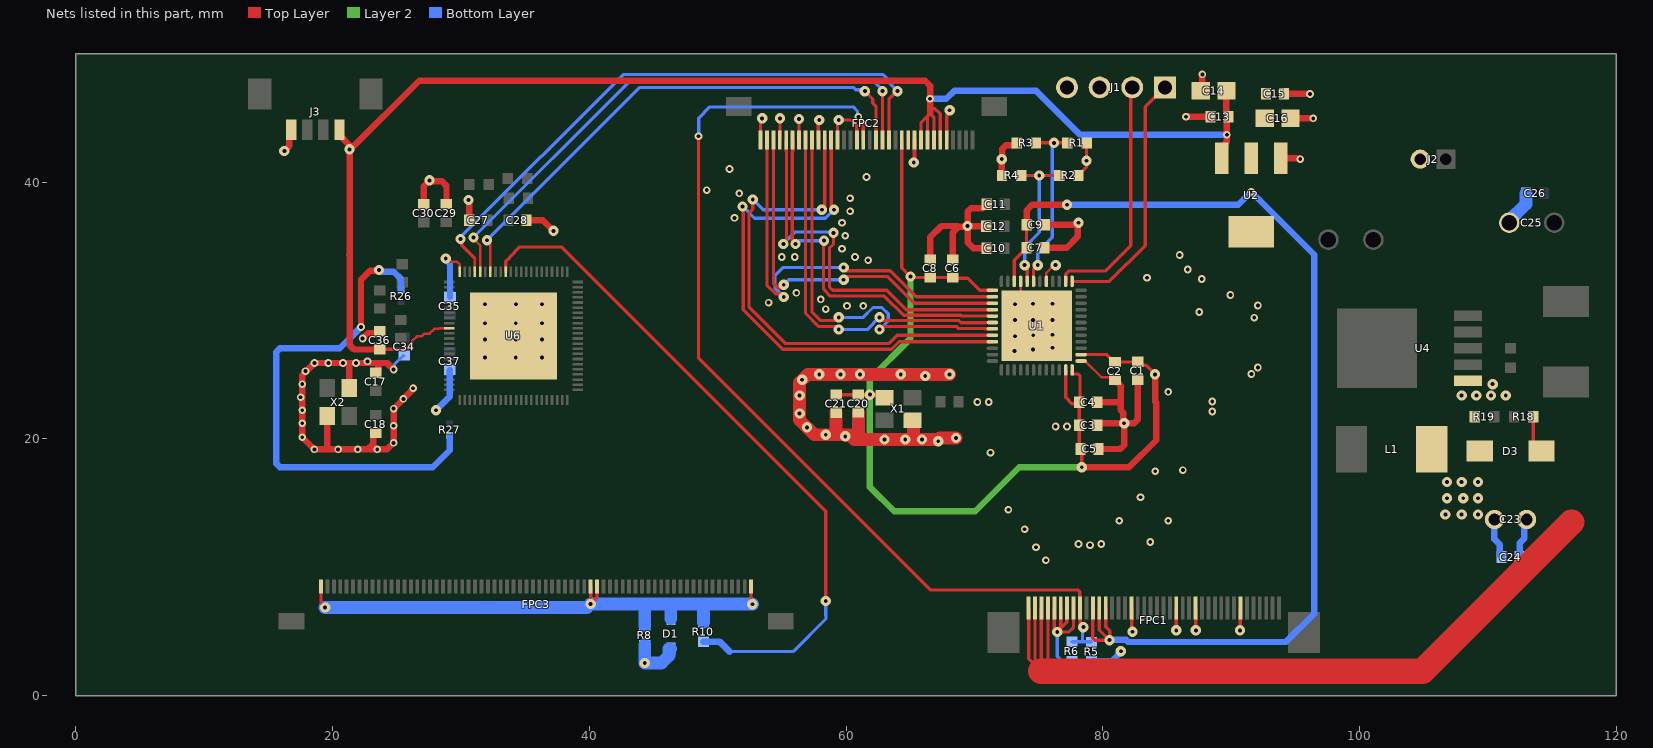
[diagram p0: the nets of this part, all layers, seen from the top]
# Altium PCB MISC71201-3.PcbDoc (part 2 of 3)
Units mm, origin at the board's own origin, x right, y up, seen from the top; angles counter-clockwise.
Board outline 120 x 50 mm, 4 copper layers (Top Layer, Layer 1, Layer 2, Bottom Layer), stack 0.603 mm thick; 69 components, 139 nets, 430 pads, 271 vias.

## Part data (continued)
C23: "Capacitance:220uF;Tolerance:±20%;Rated voltage:25V;Ripple current:510mA@100kHz;Equivalent series resistance (ESR):130mΩ@100kHz;", Equivalent Series Resistance(ESR)=130mΩ@100kHz, JLCPCB Part Class="Extended Part", LCSC Part Name="220uF ±20% 25V", Manufacturer=JIERR(捷而瑞), ManufacturerPart=ERG25V220M6X11, Operating Temperature=-40℃~+105℃, Ripple Current=510mA@100kHz, Tolerance=±20%, Voltage Rating=25V
C27: library part C0402_1u_6.3V_X5R, "SMD capacitor", PartNumber=00226021661, Value1=0.1uF/6.3V, Value2=X5R
C28 C34 C35 C36 C37: library part C0402_2.2u_6.3V_X5R, "SMD capacitor", PartNumber=002260222561, Value1=1uF/6.3V, Value2=X5R
C29 C30: library part C0603_1u_50V_X7R, "SMD capacitor", PartNumber=002260310544, Value1=4.7uF/50V, Value2=X7R
C31 C32 C33: library part C0603_1u_50V_X7R, "SMD capacitor", PartNumber=002260310544, Value1=1uF/50V, Value2=X7R
D1: library part pdyl240b_c5187140, "Reverse standoff voltage (Vrwm):24V;Clamping voltage:60V;Peak pulse power (Ppp):350W@8/20us;Breakdown voltage (VBR):26.7V;", Clamping Voltage=60V, JLCPCB Part Class="Extended Part", Junction Capacitance=1pF, LCSC Part Name="ESD 24V截止", Manufacturer=Leiditech(雷卯电子), ManufacturerPart=PDYL240B, Peak Pulse Power Dissipation (Ppp)=350W@8/20us, Reverse Leakage Current (Ir)=1uA, Reverse Stand-Off Voltage (Vrwm)=24V, Voltage - Breakdown=26.7V
D3: library part ss34_c7420365, "Diode configuration:Single;Forward voltage (Vf):550mV@3A;DC reverse voltage (Vr):40V;Rectified current:3A;", Current - Rectified=3A, JLCPCB Part Class="Extended Part", LCSC Part Name="电压:40V 电流:3A", Manufacturer=R+O(宏嘉诚), ManufacturerPart=SS34, Reverse Leakage Current (Ir)=200uA@40V, Voltage - DC Reverse(Vr)=40V, Voltage - Forward(Vf@If)=550mV@3A
FPC1: "Locking:Slide;Contact type:Bottom;Contacts:40P;Pitch:0.5mm;Mounting:Horizontal SMT;Operating temperature:-25℃~+85℃;", JLCPCB Part Class="Extended Part", LCSC Part Name="间距:0.5mm 40P 抽屉式 下接", Manufacturer=BXCONN(宝讯), ManufacturerPart=FC-05D40P11H20, Operating Temperature=-25℃~+85℃, Rated Voltage (Max)=50V
FPC2: "Locking:Flip;Contact type:Bottom;Contacts:34P;Pitch:0.5mm;Mounting:Horizontal SMT;Operating temperature:-40℃~+85℃;", Current Rating (Max)=500mA, JLCPCB Part Class="Extended Part", LCSC Part Name="FPC 翻盖式 下接 P数:34P 间距:0.5mm", Manufacturer=BXCONN(宝讯), ManufacturerPart=FC-05A34P011H20, Operating Temperature=-40℃~+85℃, Rated Voltage (Max)=50V
FPC3: "Locking:Flip;Contact type:Bottom;Contacts:68P;Pitch:0.5mm;Mounting:Horizontal SMT;Operating temperature:-25℃~+85℃;", Current Rating (Max)=500mA, JLCPCB Part Class="Extended Part", LCSC Part Name="翻盖式 下接 P数:68P 间距:0.5mm", Manufacturer=JS(钜硕电子), ManufacturerPart=AFC18-S68FIA-00, Operating Temperature=-25℃~+85℃, Rated Voltage (Max)=50V
J1: "Pin structure:1x4P;Pitch:2.54mm;Row pitch:-;Round/square pin:Square;Mounting:THT;Rows:Single;Total pins:4P;Rated current:3A;Rated voltage:1kV;Mating pin length:6mm;Insulator height:2.5mm;Tail length:3mm;Contact material:Brass;Contact plating:Gold;Operating temperature:-40℃~+105℃;Color:Black;", Color=黑色, Current Rating=3A, JLCPCB Part Class="Extended Part", LCSC Part Name="1x4P 间距:2.54mm 方针 直插", Manufacturer=hanxia(韩下), ManufacturerPart="HX PZ2.54-1x4P ZZ", Operating Temperature=-40℃~+105℃, Voltage Rating (Max)=1kV
J2: "Pin structure:1x2P;Pitch:2mm;Mounting:Right-angle THT;Series:PA;Total pins:2P;Rows:1;Pins per row:2;Row pitch:-;Rated current:3A;Contact material:Copper alloy;Contact plating:Tin;Operating temperature:-25℃~+85℃;", Color=白色, Current Rating=3A, Flame Retardant Rating=UL94V-0, JLCPCB Part Class="Extended Part", LCSC Part Name="1x2P 间距:2mm 弯插 系列:PA", Manufacturer=JST, ManufacturerPart=S02B-PASK-2(LF)(SN), Operating Temperature=-25℃~+85℃, Voltage Rating=250V
J3: "Pin structure:1x4P;Pitch:1.25mm;Mounting:Horizontal SMT;Series:PicoBlade(MX 1.25);Total pins:4P;Rows:1;Pins per row:4;Rated current:1A;Contact material:Brass;Contact plating:Tin;Operating temperature:-25℃~+85℃;", Current Rating=1A, JLCPCB Part Class="Extended Part", LCSC Part Name="1x4P 间距:1.25mm 卧贴 系列:PicoBlade(MX 1.25)", Manufacturer=LXWCONN(连兴旺电子), ManufacturerPart=MX1.25mm-4P-WT, Operating Temperature=-25℃~+85℃, Voltage Rating=125V
L1 L2: "SMD, 7x6.6x2.8mm   alloy inductor, molded inductor, high current", JLCPCB Part Class="Extended Part", LCSC Part Name="15uH ±20%", Manufacturer=cjiang(长江微电), ManufacturerPart=FXL0630-150-M
R1 R2 R3 R4 R5 R6 R7: library part Resistor
R8 R10: library part Res2, POWER=0.1W, Tolerance=1%
R9 R25: library part Res2, "SMD resistor"
R18: "Resistor type:Thin film;Resistance:86.6kΩ;Tolerance:±0.1%;Power:100mW;Temp. coefficient:±25ppm/℃;", JLCPCB Part Class="Extended Part", LCSC Part Name="薄膜电阻 86.6kΩ ±0.1% 100mW", Manufacturer=YAGEO(国巨), ManufacturerPart=RT0603BRD0786K6L, Operating Temperature Range=-55℃~+155℃, Power(Watts)=100mW, Temperature Coefficient=±25ppm/℃, Tolerance=±0.1%
R19 R20: "Resistor type:Thin film;Resistance:10kΩ;Tolerance:±0.1%;Power:100mW;Operating voltage:75V;Temp. coefficient:±25ppm/℃;", JLCPCB Part Class="Extended Part", LCSC Part Name="薄膜电阻 10kΩ ±0.1% 100mW", Manufacturer=YAGEO(国巨), ManufacturerPart=RT0603BRD0710KL, Operating Temperature=-55℃~+155℃, Power(Watts)=100mW, Temperature Coefficient=±25ppm/℃, Tolerance=±0.1%, Voltage-Supply(Max)=75V
R26 R27: library part R0402_0R_+-5%_Dup2, "SMD resistor", PartNumber=00105020003, Value1=0R, Value2=∮5%
U1: library part stm32f411ceu6, "CPU core:ARM Cortex-M4;CPU max frequency:100MHz;CPU bits:32 Bit;", JLCPCB Part Class="Extended Part", LCSC Part Name="带DSP和FPU的高性能基本型系列ARM Cortex-M4 MCU，具有512 KB Flash、100 MHz CPU和ART加速器", Manufacturer=ST(意法半导体), ManufacturerPart=STM32F411CEU6, Operating Temperature=-40℃~+85℃, Voltage - Supply=1.7V~3.6V
U2: "Output polarity:Positive;Operating voltage:12V;Output voltage:3.3V;Output current:1A;PSRR:60dB@(120Hz);Output type:Fixed;", JLCPCB Part Class="Extended Part", LCSC Part Name="3.3V 1A 12V", Manufacturer=BL(上海贝岭), ManufacturerPart=BL1117-33CX, Operating Temperature=-20℃~+125℃@(Tj), Output Current=1A, Output Voltage=3.3V, Power Supply Rejection Ratio (PSRR)=60dB@(120Hz), standby current=2mA, Voltage - Supply=12V, Voltage Dropout=1.5V@(1A)
U4: "Function:Buck-boost;Operating voltage:3.6V~32V;Output voltage:-;Output current:3A;Output type:Adjustable;", Frequency - Switching=320kHz~480kHz, JLCPCB Part Class="Extended Part", LCSC Part Name="升降压型 3A 3.6V~32V", Manufacturer=XLSEMI(芯龙), ManufacturerPart=XL6008E1, Operating Temperature=-40℃~+125℃@(TJ), Output Current=3A, Output Voltage=-, Quiescent Current=2.5mA, Voltage - Supply=3.6V~32V
U6: library part ILI2511/QFN-88/10X10_0.4_0.9, "ILITEK IC", Part Name=005122ILI2511
X1: "Frequency:26MHz;Frequency tolerance (room temp.):±10ppm;Output:CMOS;Operating voltage:1.8V~3.3V;Frequency stability:±20ppm;", Frequency Stability=±20ppm, JLCPCB Part Class="Extended Part", LCSC Part Name="YSO110TR 26MHZ 1.8V-3.3V ±10PPM -40~85℃（±20PPM) CMOS", Manufacturer=YXC(扬兴晶振), ManufacturerPart=OT322526MJBA4SL, Normal temperature Frequency Tolerance=±10ppm, Operating Temperature=-40℃~+85℃, Voltage - Supply=1.8V~3.3V
X2: "Crystal type:SMD crystal;Frequency:12MHz;Frequency tolerance (room temp.):±10ppm;Load capacitance:20pF;Frequency stability:±20ppm;", Equivalent Series Resistance(ESR)=80Ω, Frequency Stability=±20ppm, JLCPCB Part Class="Basic Part", LCSC Part Name="YSX321SL 12MHZ 4P 3225 20PF ±10PPM -40~85℃ (±20PPM)", Load Capacitance=20pF, Manufacturer=YXC(扬兴晶振), ManufacturerPart=X322512MSB4SI, Normal temperature Frequency Tolerance=±10ppm, Operating Temperature=-40℃~+85℃

## Via types
v1: diameter 0.8, hole 0.3, Top Layer to Bottom Layer, 182 vias
v2: diameter 0.6, hole 0.3, Top Layer to Bottom Layer, 89 vias

## Nets (pads, with @x,y where several pads share a name; then routed paths per layer and width w, separated by ;. In a path a pad name is that pad's centre, name@x,y a point inside that pad or via, vN(x,y) a via of type N, cw(c..) or ccw(c..) an arc to the next point about the centre after c; other vN are vias at no path point)
"1.8V for TFT": C1.2 C2.2 C3.2 C4.2 C5.1 C6.2 C8.2 C20.2 C21.2 FPC2.23 U1.13 U1.35 U1.36 U1.38 X1.4 | length 87.9
  Top Layer w0.254: C21.2@59.224,23.426 60.955,23.426 C20.2@60.97,23.442 v1(61.86,23.442) 62.75,23.442 X1.4@62.984,23.208 ; FPC2.23@64.345,43.277 64.345,33.318 v1(65.024,32.639) 65.09,32.573 C8.2@66.548,32.573 C6.2@68.326,32.573 68.387,32.512 69.469,32.512 70.419,31.562 U1.13@71.407,31.562 ; U1.35@77.107,25.362 77.107,23.223 77.597,22.733 78.051,22.733 C4.2@78.168,22.85 ; U1.36@77.608,25.362 77.608,25.059 77.62,25.047 78.077,25.047 78.232,24.892 78.232,22.914 C4.2@78.168,22.85 ; U1.38@78.306,26.561 80.321,26.561 80.9,25.982 C2.2@80.95,25.982 82.713,25.982 C1.2@82.728,25.997 83.001,25.724 83.369,25.724 v1(84.074,25.019) ; v1(78.359,17.78) 78.359,19.121 C5.1@78.273,19.207 78.174,19.307 C3.2@78.174,21.052 78.168,21.057 78.168,22.733 C4.2@78.168,22.85
  Top Layer w0.5: v1(78.359,17.78) 82.042,17.78 84.157,19.895 84.157,22.813 84.074,22.896 v1(84.074,25.019)
  Layer 2 w0.5: v1(65.024,32.639) 65.024,27.813 61.86,24.649 v1(61.86,23.442) 61.86,16.245 63.754,14.351 70.055,14.351 73.484,17.78 v1(78.359,17.78)
"3.3V for Touch&TFT": FPC2.25 J1.3 R1.1 R2.1 R5.1 R26.1 R27.1 | length 47
  Top Layer w0.254: R2.1@78.105,40.513 78.105,40.542 78.74,41.177 v1(78.74,41.656) R1.1@78.74,43.053
  Top Layer w0.3: v1(65.278,41.529) 65.345,41.596 FPC2.25@65.345,43.277
  Top Layer w0.5: v2(22.225,28.702) 22.225,32.385 22.93,33.09 23.565,33.09 v1(23.622,33.147)
  Bottom Layer w0.5: v2(22.225,28.702) 20.574,27.051 15.914,27.051 15.621,26.758 15.621,18.073 15.914,17.78 27.813,17.78 29.134,19.101 R27.1@29.134,20.262 ; v1(23.622,33.147) 23.749,33.02 24.765,33.02 25.342,32.443 R26.1@25.342,31.554 ; R5.1@79.121,2.667 80.772,2.667 80.772,2.739 81.407,3.374 v1(81.407,3.455)
"5V for BL": C13.1 C14.2 C36.2 FPC2.26 FPC2.27 FPC2.28 FPC2.29 J3.1 U2.3 U6.10 | length 115.3
  Top Layer w0.2: 25.84,27.14 26.209,27.509 26.209,27.602 26.59,27.983 26.948,27.983 27.159,28.194 27.572,28.194 27.943,28.565 28.342,28.565 28.392,28.615 U6.10@29.101,28.615
  Top Layer w0.254: C36.2@23.675,26.977 25.677,26.977 25.84,27.14 ; FPC2.26@65.845,43.277 65.845,44.636 66.345,45.136 ; FPC2.27@66.345,43.277 66.345,45.136 ; 66.548,45.72 66.929,45.72 67.345,45.304 FPC2.29@67.345,43.277 ; FPC2.28@66.845,43.277 66.845,45.042 66.548,45.339 66.345,45.136
  Top Layer w0.5: J3.1@20.544,44.066 20.544,43.666 21.336,42.874 v1(21.336,42.545) v1@21.336,42.464 ; 21.304,34.322 21.336,34.29 ; C36.2@23.675,26.977 23.498,26.977 23.476,26.955 21.686,26.955 21.336,27.305 21.336,34.29 ; 66.548,45.339 66.548,45.72 v2(66.548,46.482) 66.548,47.498 66.167,47.879 26.751,47.879 v1@21.336,42.464 ; U2.3@89.267,41.846 89.267,42.554 89.542,42.829 89.542,43.002 89.662,43.122 89.662,44.958 C13.1@89.789,45.085 89.789,45.135 89.63,45.294 C14.2@89.63,47.117 ; 21.336,34.29 v1@21.336,42.464
  Bottom Layer w0.5: v2(66.548,46.482) 67.818,46.482 68.453,47.117 74.803,47.117 78.232,43.688 v2(89.662,43.688)
+3.3V2: C7.2 C9.2 C15.1 C16.2 FPC1.11 FPC1.12 FPC1.13 U1.10 U2.2 U2.4 | length 85.1
  Top Layer w0.254: U1.10@73.107,32.261 73.107,33.892 74.055,34.841 C7.2@74.055,34.89 74.055,36.653 C9.2@74.07,36.668 ; FPC1.11@79.226,6.825 79.226,4.467 79.375,4.318 v1(80.518,4.318) ; FPC1.12@79.726,6.825 79.726,5.11 80.444,4.392 v1(80.518,4.318) ; FPC1.13@80.226,6.825 80.226,5.372 80.549,5.049 80.549,4.349 v1(80.518,4.318)
  Top Layer w0.5: C9.2@74.07,36.668 74.07,37.807 74.49,38.227 v1(77.216,38.227)
  Bottom Layer w0.5: v1(77.216,38.227) 90.551,38.227 v2(91.567,39.243) 96.464,34.346 96.464,6.384 94.258,4.178 81.995,4.178 81.836,4.337 80.537,4.337 v1(80.518,4.318)
+12V: C23.1 C24.2 D3.1 FPC1.1 FPC1.2 FPC1.3 FPC1.4 R18.2 | length 70.9
  Top Layer w0.254: FPC1.1@74.226,6.825 74.226,2.863 74.652,2.437 75.184,1.905 75.205,1.926 75.205,6.804 FPC1.3@75.226,6.825 ; 74.726,2.511 FPC1.2@74.726,6.825 ; 75.726,2.506 FPC1.4@75.726,6.825 ; R18.2@113.53,21.717 113.53,19.693 D3.1@114.163,19.06
  Top Layer w2: 75.184,1.905 76.327,1.905 ; 76.454,1.905 104.902,1.905 116.5,13.503
  Bottom Layer w0.5: C24.2@112.461,10.795 112.461,11.877 112.819,12.235 112.819,13.525 C23.1@113.01,13.716
AGND: D1.2 FPC3.1 FPC3.43 FPC3.44 FPC3.68 R8.2 R10.1 | length 43.8
  Top Layer w0.254: FPC3.1@19.11,8.484 19.11,7.179 v1(19.431,6.858) ; FPC3.43@40.11,8.484 v1(40.11,7.134) 40.61,7.634 FPC3.44@40.61,8.484 ; FPC3.68@52.61,8.484 52.61,7.207 v1(52.705,7.112)
  Bottom Layer w1: v1(19.431,6.858) 39.834,6.858 v1(40.11,7.134) 44.323,7.134 ; R8.2@44.323,5.444 44.323,7.134 ; D1.2@46.355,5.999 46.355,7.134 ; R10.1@48.895,5.715 48.895,7.007 49.022,7.134 ; v1(52.705,7.112) 52.683,7.134 49.022,7.134 ; 44.323,7.134 46.355,7.134 ; 46.355,7.134 49.022,7.134
ESD_Ring: R10.2 U6.79 | length 54.1
  Top Layer w0.254: U6.79@33.501,33.015 33.501,33.524 33.497,33.528 33.497,33.815 33.795,34.112 33.795,34.15 34.592,34.948 37.831,34.948 40.182,32.597 40.182,32.589 58.42,14.351 v1(58.42,7.366)
  Bottom Layer w0.254: 50.927,3.429 55.88,3.429 58.442,5.991 58.442,6.201 58.42,6.223 v1(58.42,7.366)
  Bottom Layer w0.5: R10.2@48.895,4.208 50.148,4.208 50.927,3.429
GND: C1.1 C2.1 C3.1 C4.1 C5.2 C6.1 C7.1 C8.1 C9.1 C10.1 C11.1 C12.2 C13.2 C14.1 C15.2 C16.1 C17.1 C18.1 C20.1 C21.1 C23.2 C24.1 C25.2 C26.1 C27.2 C28.1 C29.1 C30.1 C34.1 C35.1 C36.1 C37.1 D1.1 D3.2 FPC1.5 FPC1.6 FPC1.7 FPC1.8 FPC1.17 FPC1.24 FPC1.27 FPC1.34 FPC2.1 FPC2.4 FPC2.7 FPC2.10 FPC2.13 FPC2.16 FPC2.30 J1.4 J2.2 J3.4 L1.2 R3.2 R4.2 R6.2 R8.1 R19.2 U1.5 U1.9 U1.37 U1.49 U2.1 U4.1 U6.88 U6.89 X1.2 X2.2 X2.4 | length 189.1
  Top Layer w0.2: v1(28.829,34.036) 29.083,33.782 29.718,33.782 29.901,33.599 U6.88@29.901,33.015 ; U1.9@73.607,32.261 73.607,30.061 U1.49@74.857,28.811 ; U1.5@75.606,32.261 75.606,32.934 76.2,33.528 v1(76.327,33.528) ; U1.37@78.306,26.061 78.616,26.061 79.883,24.794 80.738,24.794 C2.1@80.95,24.582
  Top Layer w0.254: FPC2.1@53.345,43.277 53.345,44.836 v1(53.467,44.958) ; FPC2.4@54.845,43.277 54.864,43.296 v1(54.864,44.958) ; FPC2.7@56.345,43.277 v1(56.345,44.915) ; FPC2.10@57.845,43.277 57.845,44.764 v1(57.912,44.831) ; FPC2.13@59.345,43.277 59.345,44.74 v1(59.436,44.831) 60.398,44.831 60.845,44.384 FPC2.16@60.845,43.277 ; FPC2.30@67.845,43.277 67.845,45.218 68.072,45.445 v1(68.072,45.593) ; FPC1.5@76.226,6.825 76.226,5.181 v1(76.454,4.953) ; FPC1.6@76.726,6.825 76.726,5.373 76.454,5.101 v1(76.454,4.953) ; FPC1.7@77.226,6.825 77.203,6.802 77.203,5.702 v1(76.454,4.953) ; FPC1.8@77.726,6.825 77.726,5.336 77.343,4.953 v1(76.454,4.953) ; FPC1.17@82.226,6.825 82.249,6.802 82.249,5.043 v1(82.315,4.978) ; v1(85.725,5.08) FPC1.24@85.726,6.825 ; FPC1.27@87.226,6.825 87.238,6.813 87.238,5.091 v1(87.249,5.08) ; v1(90.678,5.08) 90.703,5.105 90.703,6.802 FPC1.34@90.726,6.825
  Top Layer w0.5: v1(16.256,42.418) 16.644,42.806 16.644,43.916 J3.4@16.794,44.066 ; X2.4@19.597,21.76 19.597,19.216 19.558,19.177 ; X2.2@21.297,23.96 21.297,25.869 21.336,25.908 ; v2(22.352,27.813) 22.766,28.227 23.525,28.227 C36.1@23.675,28.377 ; C18.1@23.368,20.447 23.318,20.447 23.168,20.297 23.168,19.612 22.733,19.177 ; C17.1@23.368,25.146 23.418,25.146 23.568,25.296 23.568,25.854 23.622,25.908 ; v2(24.765,25.4) 24.257,25.908 23.622,25.908 ; v2@26.289,24.003 26.289,23.876 v2(24.765,22.352) v2(24.765,19.685) 24.257,19.177 v2(23.495,19.177) 22.733,19.177 ; C30.1@27.104,38.268 27.104,39.677 v1(27.559,40.132) 27.616,40.075 28.505,40.075 28.882,39.698 C29.1@28.882,38.283 ; v1(30.607,38.608) 30.66,38.555 C27.2@30.66,37.031 ; C28.1@35.108,37.031 36.375,37.031 v1(37.211,36.195) ; C8.1@66.548,33.972 66.548,35.687 67.437,36.576 68.719,36.576 68.777,36.519 ; C6.1@68.326,33.972 68.326,36.068 68.777,36.519 ; C12.2@70.919,36.546 70.904,36.561 69.484,36.561 v1(69.469,36.576) ; C10.1@70.937,34.851 69.924,34.851 69.469,35.306 v1(69.469,36.576) ; C11.1@70.968,38.28 70.968,38.231 70.818,38.081 70.768,38.081 70.66,37.973 69.762,37.973 69.469,37.68 v1(69.469,36.576) ; R4.2@72.153,40.513 72.145,40.522 72.145,41.774 v1(72.136,41.783) 72.169,41.816 72.169,42.578 72.462,42.871 73.143,42.871 73.296,43.024 R3.2@73.296,43.053 ; C7.1@75.455,34.89 77.181,34.89 78.048,35.757 78.048,36.773 v1(78.105,36.83) ; C9.1@75.47,36.668 v1@77.862,36.668 ; C4.1@79.567,22.85 81.29,22.85 81.407,22.733 ; C3.1@79.573,21.052 79.573,21.059 79.723,21.209 v1(81.661,21.209) ; C5.2@79.672,19.207 81.368,19.207 81.661,19.5 v1(81.661,21.209) ; C2.1@80.95,24.582 80.999,24.582 81.149,24.432 81.149,24.383 81.407,24.125 81.407,22.733 ; C1.1@82.728,24.597 82.728,21.502 82.435,21.209 v1(81.661,21.209) ; v2(86.487,45.085) C13.2@88.389,45.085 ; C14.1@87.63,47.117 87.738,47.225 87.738,48.368 v2(87.757,48.387) ; U2.1@93.867,41.846 95.313,41.846 v2(95.377,41.783) ; C15.2@94.11,46.863 v2(96.139,46.863) ; C16.1@94.615,44.958 v2(96.393,44.958) ; 19.558,19.177 v2(20.447,19.177) v2(21.971,19.177) 22.733,19.177 ; 19.558,19.177 v2(18.595,19.177) v2(17.653,20.119) 17.653,24.951 v2(18.61,25.908) v2(19.685,25.908) v2(20.828,25.908) 21.336,25.908 ; 21.336,25.908 v2(21.844,25.908) 23.622,25.908 ; 68.777,36.519 69.412,36.519 v1(69.469,36.576) ; 81.407,22.733 81.407,22.225 81.604,22.028 81.604,21.266 v1(81.661,21.209)
  Top Layer w1: C21.1@59.224,22.027 59.224,20.359 59.182,20.317 ; C20.1@60.97,22.042 60.97,20.264 60.645,19.939 ; X1.2@65.184,21.458 65.263,21.379 65.263,19.939 ; v1(68.072,25.019) 57.023,25.019 56.388,24.384 56.388,21.469 57.54,20.317 59.182,20.317 ; v1(68.569,20.057) 67.301,20.057 67.183,19.939 65.263,19.939 ; 59.182,20.317 60.267,20.317 60.645,19.939 ; 60.645,19.939 v1(62.992,19.939) v1(64.613,19.939) 65.263,19.939
  Bottom Layer w0.254: v2(24.765,25.4) 24.831,25.466 24.831,25.788 25.531,26.487 C34.1@25.58,26.487 ; v1(76.454,4.953) 76.454,3.048 76.818,2.684 R6.2@77.597,2.684
  Bottom Layer w0.5: v1(28.067,22.225) 29.136,23.294 C37.1@29.136,25.359 ; v1(28.829,34.036) 28.829,33.955 29.157,33.627 C35.1@29.157,31.044 ; C23.2@110.51,13.716 110.49,13.696 110.49,12.192 110.911,11.771 110.911,10.945 C24.1@111.061,10.795
  Bottom Layer w1: R8.1@44.323,3.937 v1(44.323,2.54) 45.62,2.54 46.206,3.126 D1.1@46.206,3.655 ; D1.1@46.206,3.655 D1.1@46.355,3.655 ; C25.2@111.661,36.83 111.661,36.992 112.966,38.298 C26.1@112.966,39.116
  other v1: 106.68,14.097 107.95,14.097 109.22,14.097 106.807,15.367 108.077,15.367 109.22,15.367 106.807,16.637 107.95,16.637 109.22,16.637 67.183,19.812 65.913,19.939 59.944,20.193 58.42,20.32 56.964,20.893 56.388,21.971 56.388,23.368 107.95,23.368 109.093,23.368 110.236,23.368 111.379,23.368 110.363,24.257 56.582,24.597 66.167,24.892 57.912,25.019 59.563,25.019 61.087,25.019 64.262,25.019 31.87,26.33 34.283,26.33 36.315,26.33 73.128,26.838 74.567,26.967 76.091,27.094 31.87,27.727 34.283,27.727 36.315,27.727 73.17,27.983 74.586,28.071 76.091,28.11 31.87,28.997 34.283,28.997 36.315,28.997 73.17,29.253 74.567,29.253 76.091,29.253 31.877,30.48 34.29,30.48 36.322,30.48 73.152,30.48 74.567,30.523 76.091,30.523
  other v2: 75.565,10.541 74.803,11.557 78.999,11.717 78.105,11.811 79.883,11.811 83.698,11.971 73.914,12.954 81.285,13.622 85.095,13.622 72.644,14.478 82.943,15.452 84.084,17.476 86.238,17.559 71.247,18.923 76.327,20.955 77.216,20.955 24.765,21.018 17.653,21.209 88.524,22.131 17.653,22.225 70.231,22.86 71.12,22.86 88.529,22.903 25.527,23.114 17.526,23.241 85.095,23.655 26.289,23.939 17.653,24.257 91.572,25.052 17.907,25.273 92.08,25.56 22.733,26.035 91.797,29.438 87.508,29.878 58.42,30.099 60.071,30.353 61.341,30.353 92.08,30.386 53.975,30.607 58.039,30.861 89.933,31.2 56.134,31.369 87.705,32.454 83.444,32.545 86.619,33.18 61.722,33.909 54.991,34.163 56.007,34.163 60.706,34.163 85.984,34.323 59.69,34.798 59.944,35.814 59.69,36.83 51.308,37.211 60.325,37.719 60.325,38.735 51.689,39.116 49.149,39.37 61.595,40.386 50.927,41.021
I2C_ADDR: R1.2 R3.1 U1.7 | length 13.7
  Top Layer w0.254: U1.7@74.608,32.261 74.608,33.206 v1(74.93,33.528) ; R3.1@74.803,43.053 v1(76.2,43.053) R1.2@77.233,43.053
  Bottom Layer w0.254: v1(74.93,33.528) 74.93,34.544 76.073,35.687 v1@76.073,42.926
I2C_TYPE: R2.2 R4.1 U1.8 | length 11.7
  Top Layer w0.254: R4.1@73.66,40.513 v1(75.057,40.513) R2.2@76.598,40.513 ; v1(73.914,33.528) 73.914,33.38 74.107,33.187 U1.8@74.107,32.261
  Bottom Layer w0.254: v1(73.914,33.528) 73.914,34.925 75.057,36.068 v1(75.057,40.513)
IIC_SCL: J1.1 U1.1 | length 19.8
  Top Layer w0.254: U1.1@77.608,32.261 80.521,32.261 83.312,35.052 83.312,45.847 J1.1@84.836,47.371
IIC_SCL_TOUC_H: FPC2.20 U6.84 | length 44.1
  Top Layer w0.2: v1(30.988,35.687) 30.988,35.588 31.501,35.075 U6.84@31.501,33.015
  Top Layer w0.254: FPC2.20@62.845,43.277 v1(62.845,47.079)
  Bottom Layer w0.254: v1(30.988,35.687) 43.264,47.963 61.887,47.963 62.066,47.784 62.246,47.784 62.845,47.185 v1(62.845,47.079)
IIC_SDA: J1.2 U1.2 | length 19
  Top Layer w0.254: U1.2@77.107,32.261 77.112,32.266 77.112,32.833 77.343,33.064 80.181,33.064 82.169,35.052 82.169,47.244 J1.2@82.296,47.371
  Bottom Layer w0.254: J1.2@82.233,47.307 J1.2@82.296,47.371
IIC_SDA_TOUC_H: FPC2.21 U6.85 | length 47.2
  Top Layer w0.2: 31.097,34.05 31.101,34.046 U6.85@31.101,33.015
  Top Layer w0.254: v1(29.972,35.56) 30.076,35.456 30.076,35.071 31.097,34.05 ; FPC2.21@63.345,43.277 63.345,46.458 63.965,47.079 v1(64.008,47.079)
  Bottom Layer w0.254: v1(29.972,35.56) 29.972,35.687 42.652,48.367 62.885,48.367 63.448,47.804 63.448,47.639 v1(64.008,47.079)
INT_TOUCH: FPC2.19 U6.82 | length 41.2
  Top Layer w0.2: v1(32.033,35.462) 32.066,35.462 32.301,35.227 U6.82@32.301,33.015
  Top Layer w0.254: v1(61.468,47.079) 62.08,46.467 62.08,46.134 62.345,45.87 FPC2.19@62.345,43.277
  Bottom Layer w0.254: v1(32.033,35.462) 43.942,47.371 60.56,47.371 60.748,47.183 61.364,47.183 v1(61.468,47.079)
IO_VREF: FPC2.24
LED_EN: FPC1.9 FPC2.17 R5.2 R6.1 | length 76.8
  Top Layer w0.254: v2(48.514,43.561) 48.514,26.289 66.571,8.232 78.054,8.232 78.203,8.083 78.203,6.848 78.249,6.802 78.249,5.571 v1(78.486,5.334) ; v2(60.96,45.085) 60.96,44.991 61.345,44.606 FPC2.17@61.345,43.277
  Bottom Layer w0.254: v2(48.514,43.561) 48.533,43.58 48.533,44.979 49.401,45.847 60.579,45.847 60.894,45.533 60.894,45.151 v2(60.96,45.085) ; R6.1@77.597,4.191 78.359,4.191 ; v1(78.486,5.334) 78.412,5.26 78.412,4.244 78.359,4.191 ; R5.2@79.121,4.174 79.104,4.191 78.359,4.191
MIPI_TC_N: FPC2.9 U1.19 | length 30.7
  Top Layer w0.254: FPC2.9@57.345,43.277 57.344,42.4 57.344,29.905 58.039,29.21 59.188,29.21 v1(59.436,29.458) ; v1(62.611,28.508) 62.859,28.756 68.601,28.756 68.773,28.584 70.809,28.584 70.83,28.563 U1.19@71.407,28.563
  Bottom Layer w0.254: v1(59.436,29.458) 61.335,29.458 62.103,30.226 62.8,30.226 63.288,29.738 63.288,29.178 62.618,28.508 v1(62.611,28.508)
MIPI_TC_P: FPC2.8 U1.18 | length 29.2
  Top Layer w0.254: FPC2.8@56.845,43.277 56.844,42.4 56.844,29.763 57.851,28.756 59.188,28.756 v1(59.436,28.508) ; v1(62.611,29.458) 62.859,29.21 68.789,29.21 68.961,29.038 70.809,29.038 70.83,29.06 U1.18@71.407,29.06
  Bottom Layer w0.254: v1(59.436,28.508) 61.654,28.508 62.604,29.458 v1(62.611,29.458)
MIPI_TD0_N: FPC2.3 U1.15 | length 29.7
  Top Layer w0.254: FPC2.3@54.345,43.277 54.344,42.4 54.344,32.105 54.699,31.75 54.991,31.75 55.151,31.91 v1(55.151,31.998) ; v1(59.817,32.391) 60.065,32.639 63.246,32.639 65.277,30.608 65.353,30.608 65.4,30.562 U1.15@71.407,30.562
  Bottom Layer w0.254: v1(55.151,31.998) 55.544,32.391 v1(59.817,32.391)
MIPI_TD0_P: FPC2.2 U1.14 | length 33.2
  Top Layer w0.254: FPC2.2@53.845,43.277 53.844,42.4 53.844,31.963 54.511,31.296 54.991,31.296 55.151,31.136 v1(55.151,31.048) ; v1(59.817,33.341) 60.065,33.093 63.434,33.093 65.465,31.062 U1.14@71.407,31.062
  Bottom Layer w0.254: v1(55.151,31.048) 55.143,31.048 54.474,31.718 54.474,32.757 55.058,33.341 v1(59.817,33.341)
MIPI_TD1_N: FPC2.6 U1.17 | length 28.5
  Top Layer w0.254: FPC2.6@55.845,43.277 55.844,42.4 55.822,42.378 55.822,35.427 v1(56.07,35.179) ; v1(58.293,35.433) 58.48,35.246 58.256,35.022 58.256,31.637 58.778,31.115 62.985,31.115 64.486,29.614 68.957,29.614 69.01,29.561 U1.17@71.407,29.561
  Bottom Layer w0.254: v1(56.07,35.179) 56.324,35.433 v1(58.293,35.433)
MIPI_TD1_P: FPC2.5 U1.16 | length 30.3
  Top Layer w0.254: v1(55.12,35.179) 55.368,35.427 55.368,42.377 55.344,42.4 FPC2.5@55.345,43.277 ; v1(59.028,36.041) 59.028,35.152 58.71,34.834 58.71,31.825 58.966,31.569 63.173,31.569 64.681,30.061 U1.16@71.407,30.061
  Bottom Layer w0.254: v1(55.12,35.179) 55.12,35.186 56.044,36.11 58.96,36.11 v1(59.028,36.041)
MIPI_TD2_N: FPC2.12 U1.21 | length 42.4
  Top Layer w0.254: v1(51.943,38.1) 52.13,37.913 51.993,37.776 51.993,30.062 55.077,26.978 63.542,26.978 64.126,27.562 U1.21@71.407,27.562 ; FPC2.12@58.845,43.277 58.844,42.4 58.844,38.072 v1(59.07,37.846)
  Bottom Layer w0.254: v1(51.943,38.1) 52.874,37.169 58.4,37.169 59.07,37.839 v1(59.07,37.846)
MIPI_TD2_P: FPC2.11 U1.20 | length 40.1
  Top Layer w0.254: v1(52.742,38.645) 52.742,37.883 52.447,37.588 52.447,30.25 55.265,27.432 63.354,27.432 63.985,28.062 U1.20@71.407,28.062 ; v1(58.12,37.846) 58.344,38.071 58.344,42.4 FPC2.11@58.345,43.277
  Bottom Layer w0.254: v1(52.742,38.645) 53.541,37.846 v1(58.12,37.846)